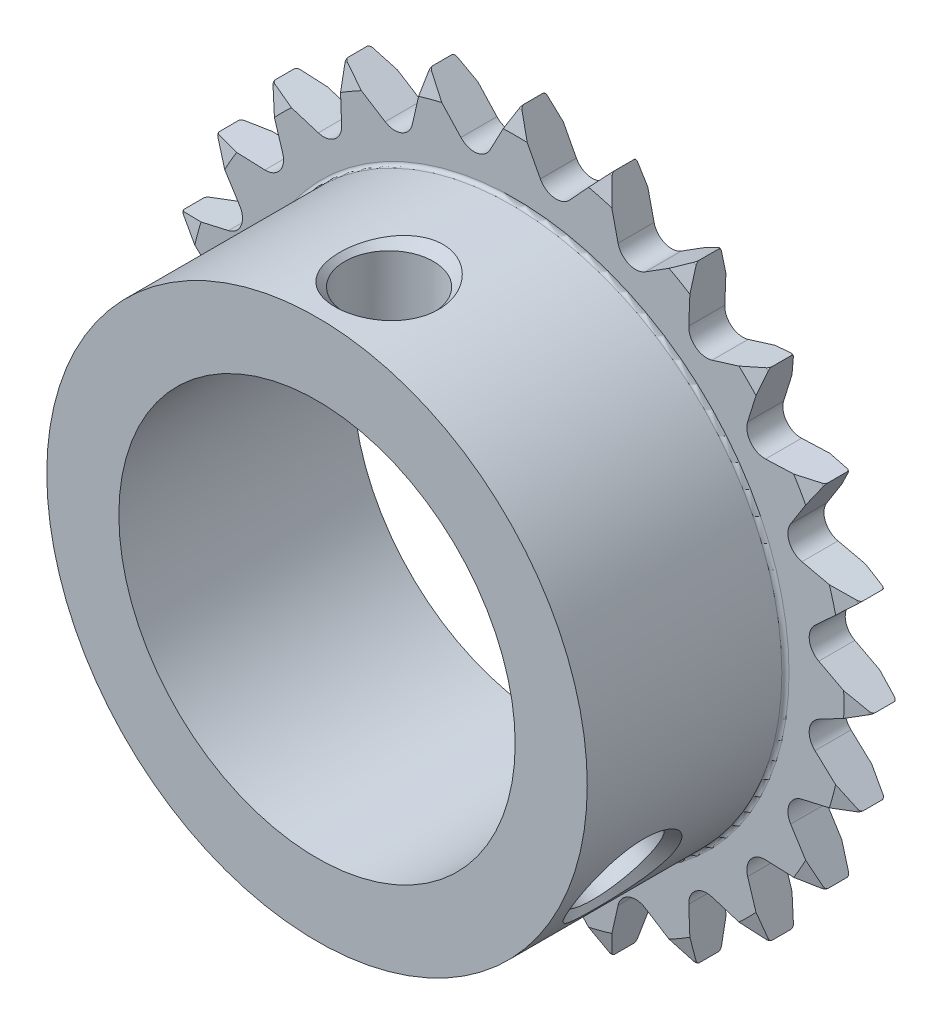
SolidWorks part; units mm, degrees
ref_plane "前视基准面" through (0, 0, 0) normal (0, 0, 1) x (1, 0, 0)
ref_plane "上视基准面" through (0, 0, 0) normal (0, 1, 0) x (1, 0, 0)
ref_plane "右视基准面" through (0, 0, 0) normal (1, 0, 0) x (0, 0, -1)
sketch "草图1" plane through (0, 0, 0) normal (1, 0, 0) x (0, 0, -1)
  line L0 (-16, 7.7) -> (-15.8, 7.5)
  line L1 (-15.8, 7.5) -> (-0.2, 7.5)
  line L2 (-0.2, 7.5) -> (0, 7.7)
  line L3 (0, 7.7) -> (0, 18.245)
  line L4 (0, 18.245) -> (-0.2966, 19.3518)
  line L5 (-0.4897, 19.5) -> (-1.5103, 19.5)
  line L6 (-1.7034, 19.3518) -> (-2, 18.245)
  line L7 (-2, 18.245) -> (-2, 15.2)
  line L8 (-2.2, 15) -> (-15.8, 15)
  line L9 (-15.8, 15) -> (-16, 14.8)
  line L10 (-16, 14.8) -> (-16, 7.7)
  line L11 (0, 0) -> (-16, 0) construction
  arc A0 (-0.2966, 19.3518) -> (-0.4897, 19.5) centre (-0.4897, 19.3) ccw
  arc A1 (-1.5103, 19.5) -> (-1.7034, 19.3518) centre (-1.5103, 19.3) ccw
  arc A2 (-2, 15.2) -> (-2.2, 15) centre (-2.2, 15.2) cw
revolve "旋转1" add sketch "草图1" angle 360 about L11
sketch "草图2" plane through (0, 0, 0) normal (0, 0, 1) x (1, 0, 0)
  line L0 (-150.3101, -119.3707) -> (151.6954, -119.3707)
  line L1 (151.6954, -119.3707) -> (151.6954, 126.7592)
  line L2 (151.6954, 126.7592) -> (-150.3101, 126.7592)
  line L3 (-150.3101, 126.7592) -> (-150.3101, -119.3707)
  line L4 (-19.5, 0) -> (-16.8512, -1.3951)
  line L5 (-16.6381, -3.0139) -> (-18.8356, -5.047)
  line L6 (-18.8356, -5.047) -> (-15.9159, -5.7089)
  line L7 (-15.2911, -7.2174) -> (-16.8875, -9.75)
  line L8 (-16.8875, -9.75) -> (-13.896, -9.6338)
  line L9 (-12.902, -10.9291) -> (-13.7886, -13.7886)
  line L10 (-13.7886, -13.7886) -> (-10.9291, -12.902)
  line L11 (-9.6338, -13.896) -> (-9.75, -16.8875)
  line L12 (-9.75, -16.8875) -> (-7.2174, -15.2911)
  line L13 (-5.7089, -15.9159) -> (-5.047, -18.8356)
  line L14 (-5.047, -18.8356) -> (-3.0139, -16.6381)
  line L15 (-1.3951, -16.8512) -> (0, -19.5)
  line L16 (0, -19.5) -> (1.3951, -16.8512)
  line L17 (3.0139, -16.6381) -> (5.047, -18.8356)
  line L18 (5.047, -18.8356) -> (5.7089, -15.9159)
  line L19 (7.2174, -15.2911) -> (9.75, -16.8875)
  line L20 (9.75, -16.8875) -> (9.6338, -13.896)
  line L21 (10.9291, -12.902) -> (13.7886, -13.7886)
  line L22 (13.7886, -13.7886) -> (12.902, -10.9291)
  line L23 (13.896, -9.6338) -> (16.8875, -9.75)
  line L24 (16.8875, -9.75) -> (15.2911, -7.2174)
  line L25 (15.9159, -5.7089) -> (18.8356, -5.047)
  line L26 (18.8356, -5.047) -> (16.6381, -3.0139)
  line L27 (16.8512, -1.3951) -> (19.5, 0)
  line L28 (19.5, 0) -> (16.8512, 1.3951)
  line L29 (16.6381, 3.0139) -> (18.8356, 5.047)
  line L30 (18.8356, 5.047) -> (15.9159, 5.7089)
  line L31 (15.2911, 7.2174) -> (16.8875, 9.75)
  line L32 (16.8875, 9.75) -> (13.896, 9.6338)
  line L33 (12.902, 10.9291) -> (13.7886, 13.7886)
  line L34 (13.7886, 13.7886) -> (10.9291, 12.902)
  line L35 (9.6338, 13.896) -> (9.75, 16.8875)
  line L36 (9.75, 16.8875) -> (7.2174, 15.2911)
  line L37 (5.7089, 15.9159) -> (5.047, 18.8356)
  line L38 (5.047, 18.8356) -> (3.0139, 16.6381)
  line L39 (1.3951, 16.8512) -> (0, 19.5)
  line L40 (0, 19.5) -> (-1.3951, 16.8512)
  line L41 (-3.0139, 16.6381) -> (-5.047, 18.8356)
  line L42 (-5.047, 18.8356) -> (-5.7089, 15.9159)
  line L43 (-7.2174, 15.2911) -> (-9.75, 16.8875)
  line L44 (-9.75, 16.8875) -> (-9.6338, 13.896)
  line L45 (-10.9291, 12.902) -> (-13.7886, 13.7886)
  line L46 (-13.7886, 13.7886) -> (-12.902, 10.9291)
  line L47 (-13.896, 9.6338) -> (-16.8875, 9.75)
  line L48 (-16.8875, 9.75) -> (-15.2911, 7.2174)
  line L49 (-15.9159, 5.7089) -> (-18.8356, 5.047)
  line L50 (-18.8356, 5.047) -> (-16.6381, 3.0139)
  line L51 (-16.8512, 1.3951) -> (-19.5, 0)
  arc A0 (-16.8512, -1.3951) -> (-16.6381, -3.0139) centre (-17.3172, -2.2799) cw
  arc A1 (-15.9159, -5.7089) -> (-15.2911, -7.2174) centre (-16.137, -6.6842) cw
  arc A2 (-13.896, -9.6338) -> (-12.902, -10.9291) centre (-13.8572, -10.633) cw
  arc A3 (-10.9291, -12.902) -> (-9.6338, -13.896) centre (-10.633, -13.8572) cw
  arc A4 (-7.2174, -15.2911) -> (-5.7089, -15.9159) centre (-6.6842, -16.137) cw
  arc A5 (-3.0139, -16.6381) -> (-1.3951, -16.8512) centre (-2.2799, -17.3172) cw
  arc A6 (1.3951, -16.8512) -> (3.0139, -16.6381) centre (2.2799, -17.3172) cw
  arc A7 (5.7089, -15.9159) -> (7.2174, -15.2911) centre (6.6842, -16.137) cw
  arc A8 (9.6338, -13.896) -> (10.9291, -12.902) centre (10.633, -13.8572) cw
  arc A9 (12.902, -10.9291) -> (13.896, -9.6338) centre (13.8572, -10.633) cw
  arc A10 (15.2911, -7.2174) -> (15.9159, -5.7089) centre (16.137, -6.6842) cw
  arc A11 (16.6381, -3.0139) -> (16.8512, -1.3951) centre (17.3172, -2.2799) cw
  arc A12 (16.8512, 1.3951) -> (16.6381, 3.0139) centre (17.3172, 2.2799) cw
  arc A13 (15.9159, 5.7089) -> (15.2911, 7.2174) centre (16.137, 6.6842) cw
  arc A14 (13.896, 9.6338) -> (12.902, 10.9291) centre (13.8572, 10.633) cw
  arc A15 (10.9291, 12.902) -> (9.6338, 13.896) centre (10.633, 13.8572) cw
  arc A16 (7.2174, 15.2911) -> (5.7089, 15.9159) centre (6.6842, 16.137) cw
  arc A17 (3.0139, 16.6381) -> (1.3951, 16.8512) centre (2.2799, 17.3172) cw
  arc A18 (-1.3951, 16.8512) -> (-3.0139, 16.6381) centre (-2.2799, 17.3172) cw
  arc A19 (-5.7089, 15.9159) -> (-7.2174, 15.2911) centre (-6.6842, 16.137) cw
  arc A20 (-9.6338, 13.896) -> (-10.9291, 12.902) centre (-10.633, 13.8572) cw
  arc A21 (-12.902, 10.9291) -> (-13.896, 9.6338) centre (-13.8572, 10.633) cw
  arc A22 (-15.2911, 7.2174) -> (-15.9159, 5.7089) centre (-16.137, 6.6842) cw
  arc A23 (-16.6381, 3.0139) -> (-16.8512, 1.3951) centre (-17.3172, 2.2799) cw
extrude "切除-拉伸1" cut sketch "草图2" along normal blind 2
ref_plane "基准面4" through (0, 0, 9) normal (0, 0, 1) x (1, 0, 0)
sketch "草图3" plane through (0, 0, 9) normal (0, 0, 1) x (1, 0, 0)
  line L0 (0, 2.3) -> (-3, 2.3)
  line L1 (-3, 2.3) -> (-3, 9.8)
  line L2 (-3, 9.8) -> (-2.4585, 10.3415)
  line L3 (-2.4585, 10.3415) -> (-2.4585, 14.4585)
  line L4 (-2.4585, 14.4585) -> (-3, 15)
  line L5 (-3, 15) -> (-3, 22.5)
  line L6 (-3, 22.5) -> (0, 22.5)
  line L7 (0, 22.5) -> (0, 2.3)
  line L8 (0, 15) -> (0, 9.8) construction
revolve "切除-旋转1" cut sketch "草图3" angle 360 about L8
cosmetic thread "装饰螺纹线1" parameters "D1"=4.6585, "D2"=6
sketch "草图4" plane through (0, 0, 9) normal (0, 0, 1) x (1, 0, 0)
  line L0 (0, 0) -> (1.5, 2.5981)
  line L1 (1.5, 2.5981) -> (7.9952, -1.1519)
  line L2 (7.9952, -1.1519) -> (8.1934, -1.8916)
  line L3 (8.1934, -1.8916) -> (13.7507, -5.1001)
  line L4 (13.7507, -5.1001) -> (14.4904, -4.9019)
  line L5 (14.4904, -4.9019) -> (20.9856, -8.6519)
  line L6 (20.9856, -8.6519) -> (19.4856, -11.25)
  line L7 (19.4856, -11.25) -> (0, 0)
  line L8 (12.9904, -7.5) -> (6.4952, -3.75) construction
revolve "切除-旋转2" cut sketch "草图4" angle 360 about L8
cosmetic thread "装饰螺纹线2" parameters "D1"=6.9585, "D2"=6
sketch "草图5" plane through (0, 0, 0) normal (0, 1, 0) x (1, 0, 0)
  line L1 (-15.7669, -16) -> (17.9123, -16)
  line L2 (-15.7669, -16) -> (-15.7669, -13)
  line L3 (-15.7669, -13) -> (17.9123, -13)
  line L4 (17.9123, -16) -> (17.9123, -13)
  dimension "D1" = 3
extrude "切除-拉伸2" cut sketch "草图5" against normal through all and the other way through all
sketch "草图6" plane through (0, 0, 0) normal (0, 0, -1) x (-1, 0, 0)
  circle A0 centre (0, 0) radius 11
  dimension "D1" = 22
extrude "切除-拉伸3" cut sketch "草图6" against normal through all
